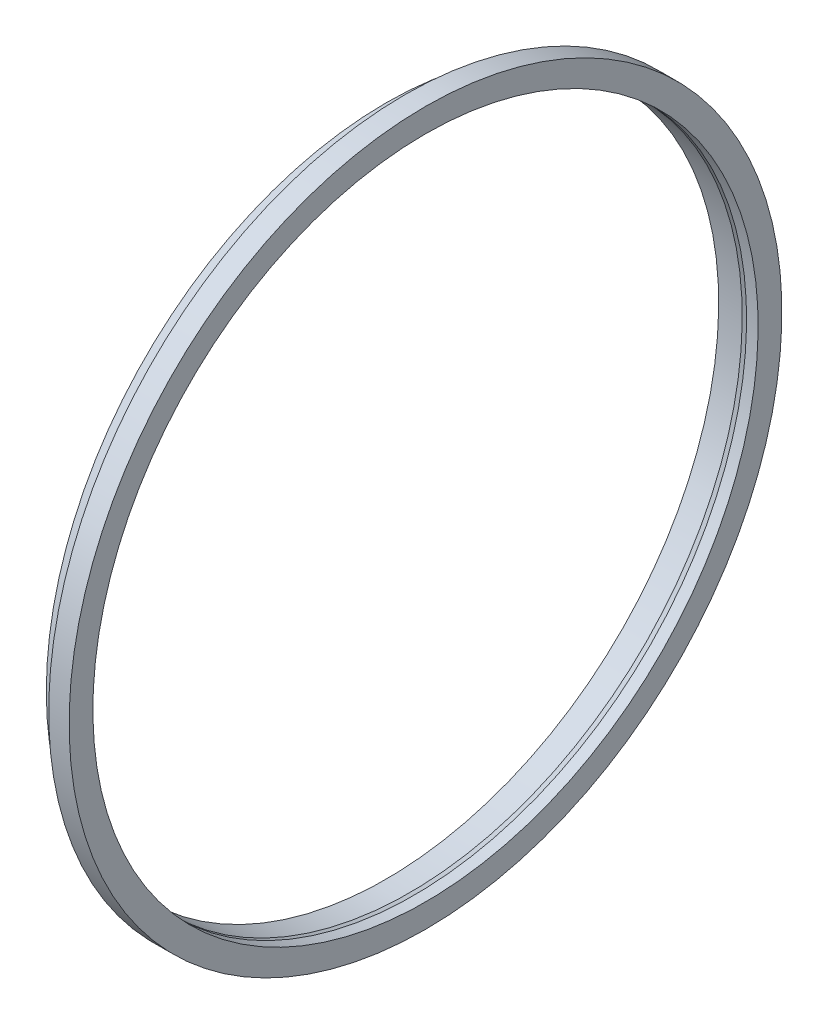
from build123d import *


with BuildPart() as part:
    # Sketch1 → Revolve1 (revolve)
    with BuildSketch(Plane.XY):
        Polygon((-70, 70), (-70, 71.5), (-66, 72.65), (-66, 75), (-61.7, 75), (-61.7, 70), (-64.127855471, 70), (-64.127855471, 70.546927726), (-65.050124916, 70), align=None)
    revolve(axis=Axis((0, 0, 0), (-1, 0, 0)))


solid = part.part
